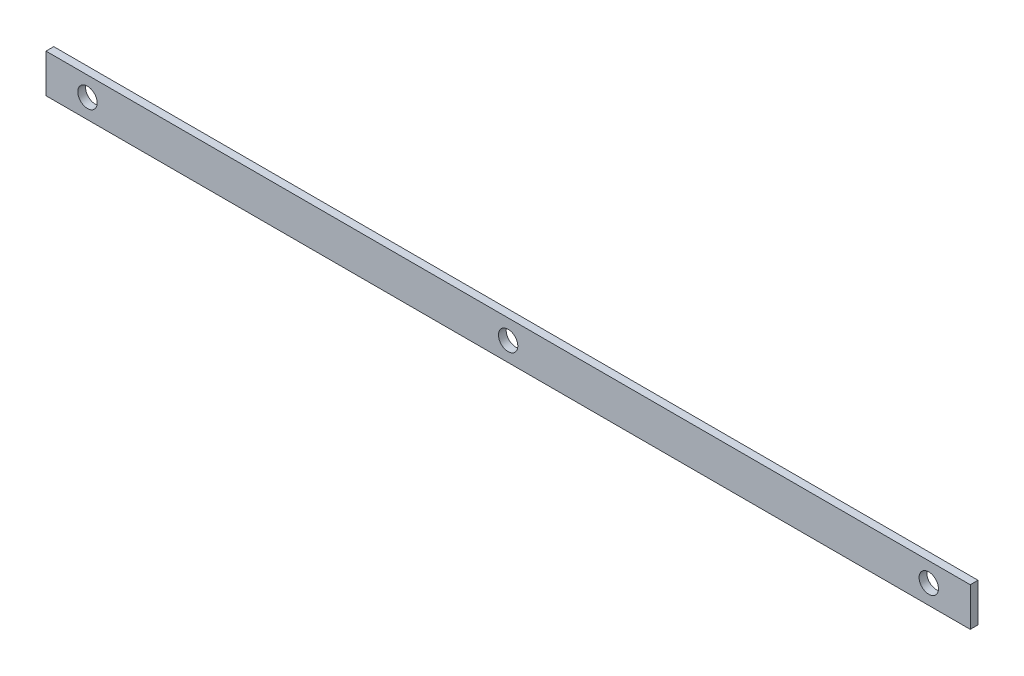
from build123d import *

# Parameters (mm, degrees)
SKETCH1_W           = 119.309628318
SKETCH1_H           = 4.994236566
BOSS_EXTRUDE1_DEPTH = 1
SKETCH2_R           = 1.25
CUT_EXTRUDE1_DEPTH  = 1


with BuildPart() as part:
    # Sketch1 → Boss-Extrude1 (new body)
    with BuildSketch(Plane.XY):
        with Locations((0, 59.58360497)):
            Rectangle(SKETCH1_W, SKETCH1_H)
    extrude(amount=BOSS_EXTRUDE1_DEPTH)

    # Sketch2 → Cut-Extrude1 (cut)
    with BuildSketch(Plane.XY.offset(1)):
        with Locations((-54.300260115, 59.58360497)):
            Circle(SKETCH2_R)
        with Locations((0, 59.560111084)):
            Circle(SKETCH2_R)
        with Locations((54.300260115, 59.58360497)):
            Circle(SKETCH2_R)
    extrude(amount=-CUT_EXTRUDE1_DEPTH, mode=Mode.SUBTRACT)


solid = part.part
